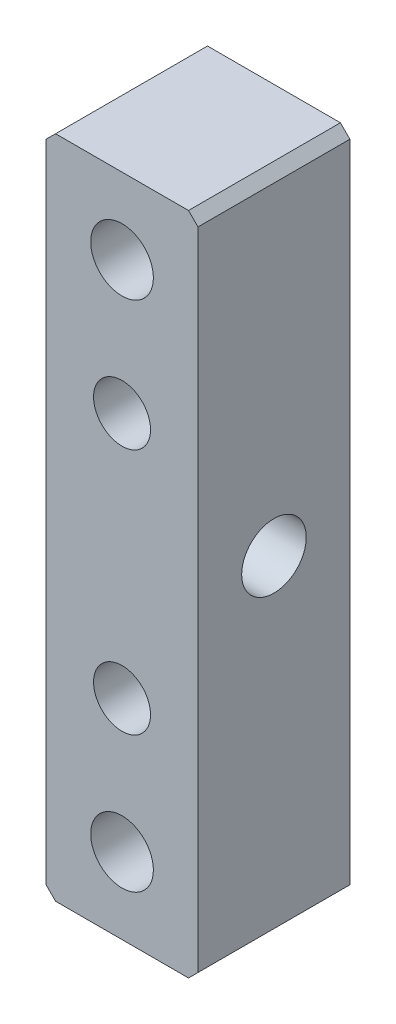
from build123d import *

# Parameters (mm, degrees)
SKETCH1_W                    = 16
SKETCH1_H                    = 70
EXTRUDE_THIN1_DEPTH          = 16
CHAMFER1_SIZE                = 1
SIZE_MM_BLIND_DOWEL_HOLE_1_D = 6
M8_TAPPED_HOLE1_D            = 6.8
M6_CLEARANCE_HOLE1_D         = 6.6


with BuildPart() as part:
    # Sketch1 → Extrude-Thin1 (new body)
    with BuildSketch(Plane.XY):
        with Locations((-8, 35)):
            Rectangle(SKETCH1_W, SKETCH1_H)
    extrude(amount=EXTRUDE_THIN1_DEPTH)

    # Chamfer1
    chamfer1_edges = [part.edges().sort_by_distance(p)[0] for p in [
        (-16, 70, 8),
        (0, 70, 8),
        (0, 0, 8),
        (-16, 0, 8),
    ]]
    chamfer(chamfer1_edges, length=CHAMFER1_SIZE)

    # Size mm blind dowel hole 1 (through all)
    with Locations(Plane.XY.offset(16)):
        with Locations((-8, 48), (-8, 22)):
            Hole(SIZE_MM_BLIND_DOWEL_HOLE_1_D / 2)

    # M8 Tapped Hole1 (through all)
    with Locations(Plane.ZY.offset(16)):
        with Locations((8, 35)):
            Hole(M8_TAPPED_HOLE1_D / 2)

    # M6 Clearance Hole1 (through all)
    with Locations(Plane.XY.offset(16)):
        with Locations((-8, 62), (-8, 8)):
            Hole(M6_CLEARANCE_HOLE1_D / 2)


solid = part.part
